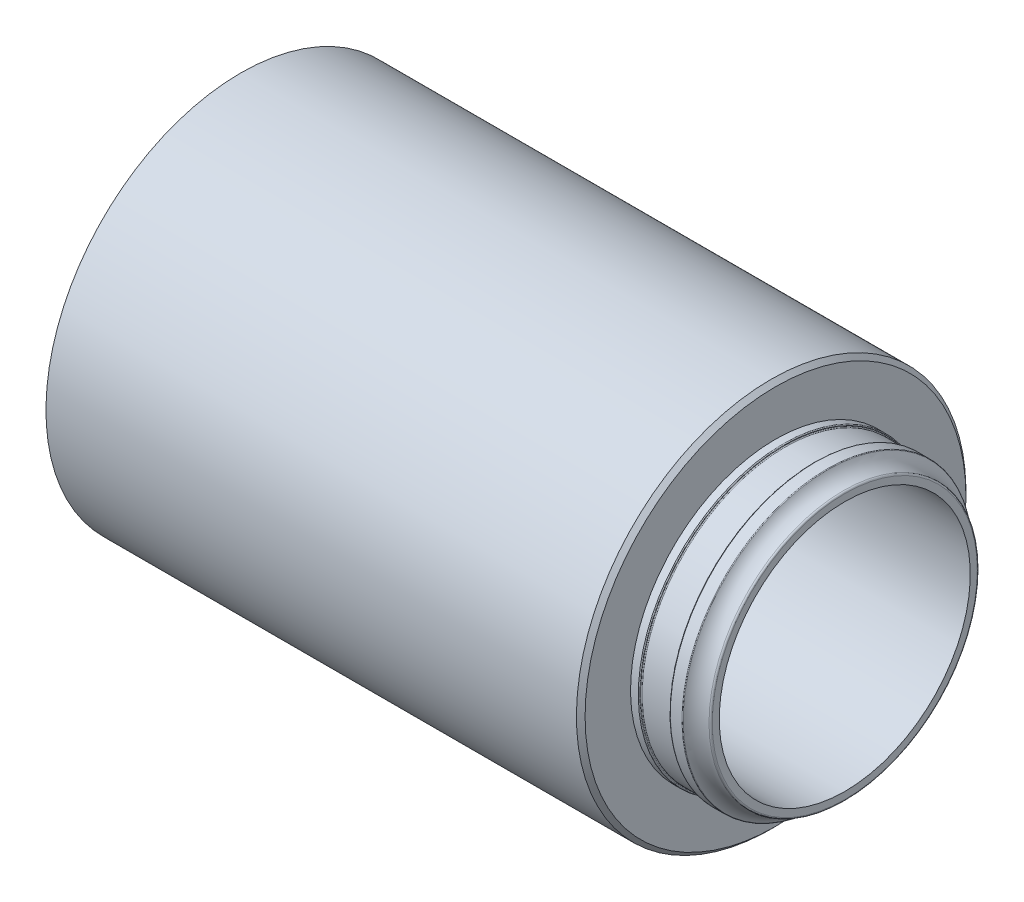
SolidWorks part; units mm, degrees
ref_plane "Front Plane" through (0, 0, 0) normal (0, 0, 1) x (1, 0, 0)
ref_plane "Top Plane" through (0, 0, 0) normal (0, 1, 0) x (1, 0, 0)
ref_plane "Right Plane" through (0, 0, 0) normal (1, 0, 0) x (0, 0, -1)
other "Configuration Table"
sketch "Sketch1" plane through (0, 0, 0) normal (0, 0, 1) x (1, 0, 0)
  line L0 (597.1745, 0) -> (234.8282, 0) construction
  line L1 (437.2643, 33.5) -> (434.5845, 33.5)
  line L2 (427.1845, 33.5) -> (425.3845, 33.5)
  line L3 (434.1845, 33) -> (427.5845, 33)
  line L4 (424.3845, 45) -> (411.8245, 45)
  line L5 (411.8245, 45) -> (391.8245, 45)
  line L6 (391.8245, 45) -> (301.8245, 45)
  line L7 (301.8245, 45) -> (301.8245, 29)
  line L8 (441.3845, 30.6158) -> (441.3845, 29)
  line L9 (425.3845, 44) -> (425.3845, 33.5)
  line L10 (427.3845, 33.3) -> (427.3845, 33.2)
  line L11 (434.3845, 33.3) -> (434.3845, 33.2)
  line L12 (424.3845, 45) -> (425.3845, 44)
  line L13 (301.8245, 29) -> (441.3845, 29)
  arc A0 (427.3845, 33.2) -> (427.5845, 33) centre (427.5845, 33.2) ccw
  arc A1 (427.3845, 33.3) -> (427.1845, 33.5) centre (427.1845, 33.3) ccw
  arc A2 (434.1845, 33) -> (434.3845, 33.2) centre (434.1845, 33.2) ccw
  arc A3 (434.5845, 33.5) -> (434.3845, 33.3) centre (434.5845, 33.3) ccw
  arc A4 (437.4397, 33.3961) -> (441.0257, 31.0137) centre (441.5031, 35.6223) ccw
  arc A5 (437.4397, 33.3961) -> (437.2643, 33.5) centre (437.2643, 33.3) ccw
  arc A6 (441.3845, 30.6158) -> (441.0257, 31.0137) centre (440.9845, 30.6158) ccw
revolve "Revolve1" add sketch "Sketch1" angle 360 about L0
